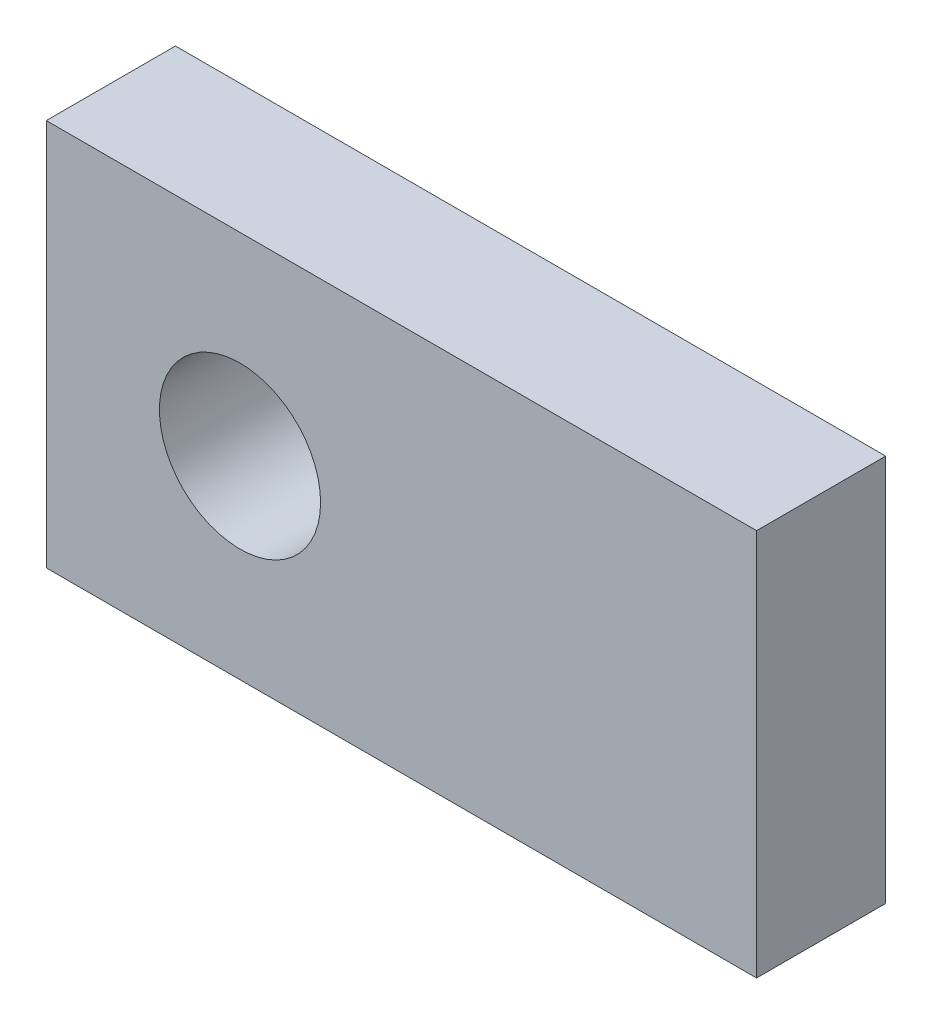
from build123d import *

# Parameters (mm, degrees)
SKETCH1_W           = 34.925
SKETCH1_H           = 19.05
SKETCH1_R           = 3.9624
BOSS_EXTRUDE1_DEPTH = 6.35


with BuildPart() as part:
    # Sketch1 → Boss-Extrude1 (new body)
    with BuildSketch(Plane.XY):
        with Locations((17.4625, 9.525)):
            Rectangle(SKETCH1_W, SKETCH1_H)
        with Locations((9.525, 9.525)):
            Circle(SKETCH1_R, mode=Mode.SUBTRACT)
    extrude(amount=BOSS_EXTRUDE1_DEPTH)


solid = part.part
